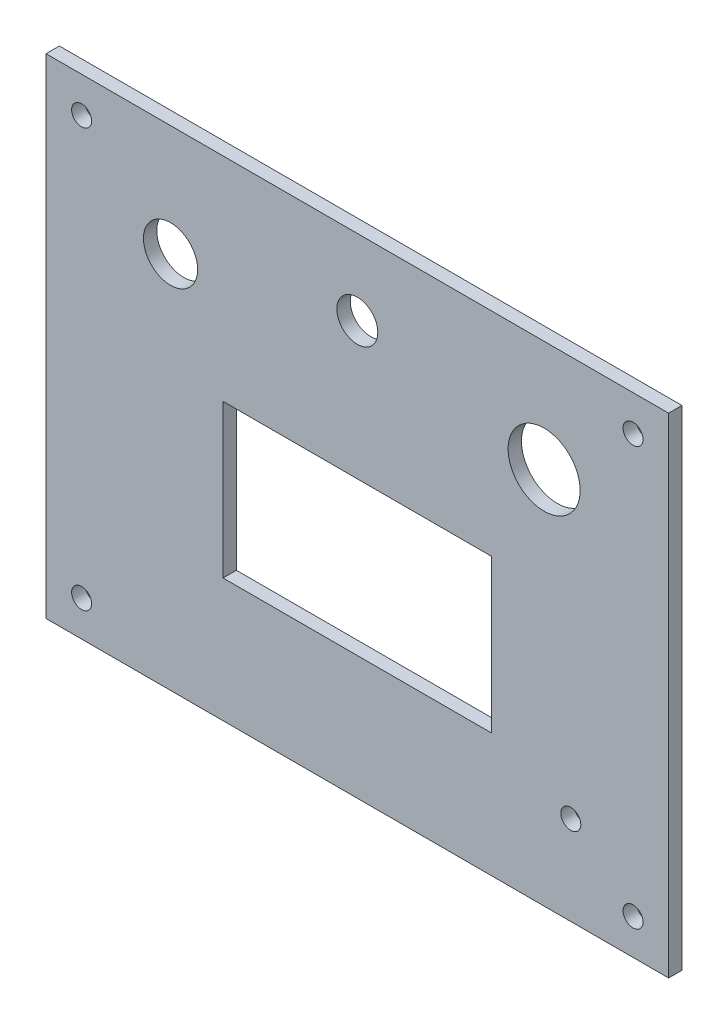
from build123d import *

# Parameters (mm, degrees)
SKETCH_1_W      = 140
SKETCH_1_H      = 110
SKETCH_1_R      = 2.25
SKETCH_1_R_2    = 6.1
SKETCH_1_R_3    = 8.1
SKETCH_1_R_4    = 4.6
SKETCH_1_W_2    = 60.4
SKETCH_1_H_2    = 34.4
EXTRUDE_1_DEPTH = 1.5


with BuildPart() as part:
    # 草图1 → 凸台-拉伸1 (new, symmetric)
    with BuildSketch(Plane.XY):
        Rectangle(SKETCH_1_W, SKETCH_1_H)
        with Locations((-62, -47)):
            Circle(SKETCH_1_R, mode=Mode.SUBTRACT)
        with Locations((-62, 47)):
            Circle(SKETCH_1_R, mode=Mode.SUBTRACT)
        with Locations((62, -47)):
            Circle(SKETCH_1_R, mode=Mode.SUBTRACT)
        with Locations((62, 47)):
            Circle(SKETCH_1_R, mode=Mode.SUBTRACT)
        with Locations((-42, 30)):
            Circle(SKETCH_1_R_2, mode=Mode.SUBTRACT)
        with Locations((42, 30)):
            Circle(SKETCH_1_R_3, mode=Mode.SUBTRACT)
        with Locations((0, 38)):
            Circle(SKETCH_1_R_4, mode=Mode.SUBTRACT)
        with Locations((48, -35)):
            Circle(SKETCH_1_R, mode=Mode.SUBTRACT)
        with Locations((0, -10)):
            Rectangle(SKETCH_1_W_2, SKETCH_1_H_2, mode=Mode.SUBTRACT)
    extrude(amount=EXTRUDE_1_DEPTH, both=True)


solid = part.part
